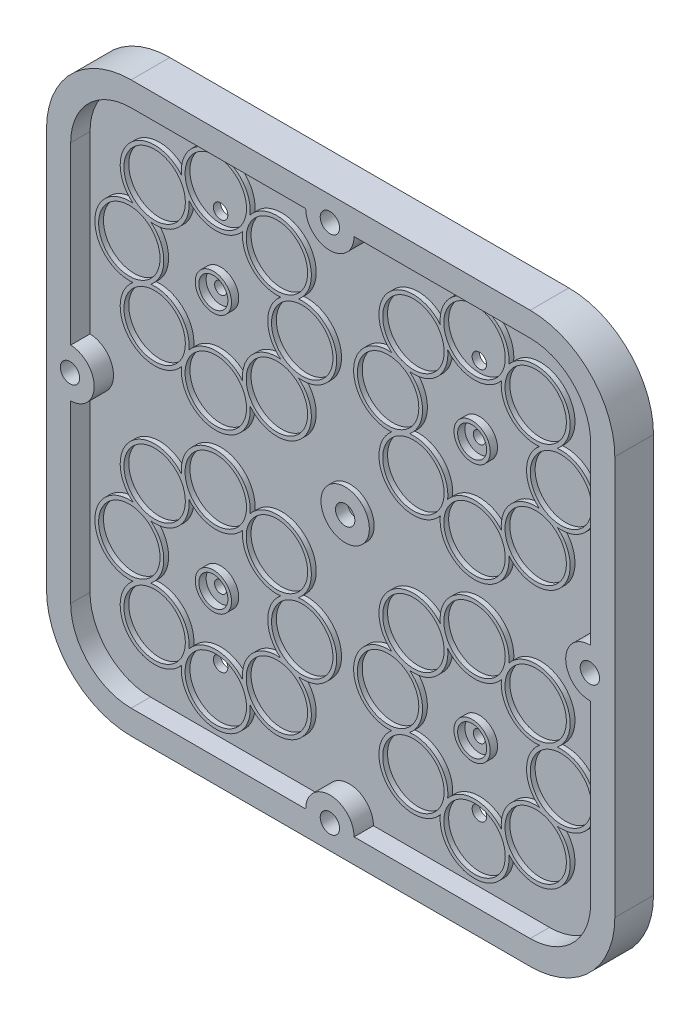
from build123d import *

# Parameters (mm, degrees)
SKETCH1_R           = 4
SKETCH1_R_2         = 2.5
BOSS_EXTRUDE1_DEPTH = 3
SKETCH2_R           = 4
BOSS_EXTRUDE2_DEPTH = 8
SKETCH3_R           = 10
SKETCH3_R_2         = 4
BOSS_EXTRUDE3_DEPTH = 2
SKETCH4_R           = 12.7
BOSS_EXTRUDE4_DEPTH = 2
SKETCH5_R           = 7.5
SKETCH5_R_2         = 6
BOSS_EXTRUDE5_DEPTH = 3
SKETCH6_R           = 3
CUT_EXTRUDE1_DEPTH  = 10
BOSS_EXTRUDE6_START = 4
SKETCH7_R           = 19
SKETCH7_R_2         = 7.5
BOSS_EXTRUDE6_DEPTH = 4
SKETCH8_R           = 14.5
SKETCH8_R_2         = 9.5
BOSS_EXTRUDE7_DEPTH = 6


with BuildPart() as part:
    # Sketch1 → Boss-Extrude1 (new body)
    with BuildSketch(Plane.XY):
        with BuildLine():
            Line((35, 0), (200, 0))
            ThreePointArc((200, 0), (224.748737342, 10.251262658), (235, 35))
            Line((235, 35), (235, 200))
            ThreePointArc((235, 200), (224.748737342, 224.748737342), (200, 235))
            Line((200, 235), (35, 235))
            ThreePointArc((35, 235), (10.251262658, 224.748737342), (0, 200))
            Line((0, 200), (0, 35))
            ThreePointArc((0, 35), (10.251262658, 10.251262658), (35, 0))
        make_face()
        with Locations((117.5, 225)):
            Circle(SKETCH1_R, mode=Mode.SUBTRACT)
        with Locations((117.5, 10)):
            Circle(SKETCH1_R, mode=Mode.SUBTRACT)
        with Locations((117.5, 117.5)):
            Circle(SKETCH1_R, mode=Mode.SUBTRACT)
        with Locations((225, 117.5)):
            Circle(SKETCH1_R, mode=Mode.SUBTRACT)
        with Locations((10, 117.5)):
            Circle(SKETCH1_R, mode=Mode.SUBTRACT)
        with Locations((64, 171)):
            Circle(SKETCH1_R_2, mode=Mode.SUBTRACT)
        with Locations((171, 171)):
            Circle(SKETCH1_R_2, mode=Mode.SUBTRACT)
        with Locations((171, 64)):
            Circle(SKETCH1_R_2, mode=Mode.SUBTRACT)
        with Locations((64, 64)):
            Circle(SKETCH1_R_2, mode=Mode.SUBTRACT)
    extrude(amount=BOSS_EXTRUDE1_DEPTH)

    # Sketch2 → Boss-Extrude2 (add, symmetric)
    with BuildSketch(Plane.XY.offset(3)):
        with BuildLine():
            Line((235, 35), (235, 200))
            ThreePointArc((235, 200), (224.748737342, 224.748737342), (200, 235))
            Line((200, 235), (35, 235))
            ThreePointArc((35, 235), (10.251262658, 224.748737342), (0, 200))
            Line((0, 200), (0, 35))
            ThreePointArc((0, 35), (10.251262658, 10.251262658), (35, 0))
            Line((35, 0), (200, 0))
            ThreePointArc((200, 0), (224.748737342, 10.251262658), (235, 35))
        make_face()
        with Locations((117.185983795, 225.007361775)):
            Circle(SKETCH2_R, mode=Mode.SUBTRACT)
        with Locations((224.685983795, 117.507361775)):
            Circle(SKETCH2_R, mode=Mode.SUBTRACT)
        with Locations((117.185983795, 10.007361775)):
            Circle(SKETCH2_R, mode=Mode.SUBTRACT)
        with Locations((9.72235037, 117.506509199)):
            Circle(SKETCH2_R, mode=Mode.SUBTRACT)
        with BuildLine():
            Line((200, 225), (127.185981085, 225))
            ThreePointArc((127.185981085, 225), (117.185983795, 215.007361775), (107.185986504, 225))
            Line((107.185986504, 225), (35, 225))
            ThreePointArc((35, 225), (17.32233047, 217.67766953), (10, 200))
            Line((10, 200), (10, 127.50265399))
            ThreePointArc((10, 127.50265399), (19.72235037, 117.506509199), (10, 107.510364408))
            Line((10, 107.510364408), (10, 35))
            ThreePointArc((10, 35), (17.32233047, 17.32233047), (35, 10))
            Line((35, 10), (107.185986504, 10))
            ThreePointArc((107.185986504, 10), (117.185983795, 20.007361775), (127.185981085, 10))
            Line((127.185981085, 10), (200, 10))
            ThreePointArc((200, 10), (217.67766953, 17.32233047), (225, 35))
            Line((225, 35), (225, 107.5122933))
            ThreePointArc((225, 107.5122933), (214.685983795, 117.507361775), (225, 127.50243025))
            Line((225, 127.50243025), (225, 200))
            ThreePointArc((225, 200), (217.67766953, 217.67766953), (200, 225))
        make_face(mode=Mode.SUBTRACT)
    extrude(amount=BOSS_EXTRUDE2_DEPTH, both=True)

    # Sketch3 → Boss-Extrude3 (add)
    with BuildSketch(Plane.XY.offset(3)):
        with Locations((117.5, 117.5)):
            Circle(SKETCH3_R)
        with Locations((117.5, 117.5)):
            Circle(SKETCH3_R_2, mode=Mode.SUBTRACT)
    extrude(amount=BOSS_EXTRUDE3_DEPTH)

    # Sketch4 → Boss-Extrude4 (add)
    # profile 1 of 4: a face of its own
    with BuildSketch(Plane.XY.offset(3)):
        with BuildLine():
            ThreePointArc((136.802142668, 185.165216311), (121, 171), (136.802142668, 156.834783689))
            ThreePointArc((136.802142668, 156.834783689), (135.644660941, 135.644660941), (156.834783689, 136.802142668))
            ThreePointArc((156.834783689, 136.802142668), (171, 121), (185.165216311, 136.802142668))
            ThreePointArc((185.165216311, 136.802142668), (206.355339059, 135.644660941), (205.197857332, 156.834783689))
            ThreePointArc((205.197857332, 156.834783689), (221, 171), (205.197857332, 185.165216311))
            ThreePointArc((205.197857332, 185.165216311), (206.355339059, 206.355339059), (185.165216311, 205.197857332))
            ThreePointArc((185.165216311, 205.197857332), (171, 221), (156.834783689, 205.197857332))
            ThreePointArc((156.834783689, 205.197857332), (135.644660941, 206.355339059), (136.802142668, 185.165216311))
        make_face()
        with Locations((171, 206.75)):
            Circle(SKETCH4_R, mode=Mode.SUBTRACT)
        with Locations((145.720932573, 196.279067427)):
            Circle(SKETCH4_R, mode=Mode.SUBTRACT)
        with Locations((135.25, 171)):
            Circle(SKETCH4_R, mode=Mode.SUBTRACT)
        with Locations((145.720932573, 145.720932573)):
            Circle(SKETCH4_R, mode=Mode.SUBTRACT)
        with Locations((171, 135.25)):
            Circle(SKETCH4_R, mode=Mode.SUBTRACT)
        with Locations((196.279067427, 145.720932573)):
            Circle(SKETCH4_R, mode=Mode.SUBTRACT)
        with Locations((206.75, 171)):
            Circle(SKETCH4_R, mode=Mode.SUBTRACT)
        with Locations((196.279067427, 196.279067427)):
            Circle(SKETCH4_R, mode=Mode.SUBTRACT)
        with BuildLine():
            ThreePointArc((159.886148884, 197.831210095), (171, 192.5), (182.113851116, 197.831210095))
            ThreePointArc((182.113851116, 197.831210095), (186.202795796, 186.202795796), (197.831210095, 182.113851116))
            ThreePointArc((197.831210095, 182.113851116), (192.5, 171), (197.831210095, 159.886148884))
            ThreePointArc((197.831210095, 159.886148884), (186.202795796, 155.797204204), (182.113851116, 144.168789905))
            ThreePointArc((182.113851116, 144.168789905), (171, 149.5), (159.886148884, 144.168789905))
            ThreePointArc((159.886148884, 144.168789905), (155.797204204, 155.797204204), (144.168789905, 159.886148884))
            ThreePointArc((144.168789905, 159.886148884), (149.5, 171), (144.168789905, 182.113851116))
            ThreePointArc((144.168789905, 182.113851116), (155.797204204, 186.202795796), (159.886148884, 197.831210095))
        make_face(mode=Mode.SUBTRACT)
    # profile 2 of 4: a face of its own
    with BuildSketch(Plane.XY.offset(3)):
        with BuildLine():
            ThreePointArc((185.165216311, 98.197857332), (171, 114), (156.834783689, 98.197857332))
            ThreePointArc((156.834783689, 98.197857332), (135.644660941, 99.355339059), (136.802142668, 78.165216311))
            ThreePointArc((136.802142668, 78.165216311), (121, 64), (136.802142668, 49.834783689))
            ThreePointArc((136.802142668, 49.834783689), (135.644660941, 28.644660941), (156.834783689, 29.802142668))
            ThreePointArc((156.834783689, 29.802142668), (171, 14), (185.165216311, 29.802142668))
            ThreePointArc((185.165216311, 29.802142668), (206.355339059, 28.644660941), (205.197857332, 49.834783689))
            ThreePointArc((205.197857332, 49.834783689), (221, 64), (205.197857332, 78.165216311))
            ThreePointArc((205.197857332, 78.165216311), (206.355339059, 99.355339059), (185.165216311, 98.197857332))
        make_face()
        with Locations((171, 99.75)):
            Circle(SKETCH4_R, mode=Mode.SUBTRACT)
        with Locations((145.720932573, 89.279067427)):
            Circle(SKETCH4_R, mode=Mode.SUBTRACT)
        with Locations((135.25, 64)):
            Circle(SKETCH4_R, mode=Mode.SUBTRACT)
        with Locations((145.720932573, 38.720932573)):
            Circle(SKETCH4_R, mode=Mode.SUBTRACT)
        with Locations((171, 28.25)):
            Circle(SKETCH4_R, mode=Mode.SUBTRACT)
        with Locations((196.279067427, 38.720932573)):
            Circle(SKETCH4_R, mode=Mode.SUBTRACT)
        with Locations((206.75, 64)):
            Circle(SKETCH4_R, mode=Mode.SUBTRACT)
        with Locations((196.279067427, 89.279067427)):
            Circle(SKETCH4_R, mode=Mode.SUBTRACT)
        with BuildLine():
            ThreePointArc((144.168789905, 75.113851116), (155.797204204, 79.202795796), (159.886148884, 90.831210095))
            ThreePointArc((159.886148884, 90.831210095), (171, 85.5), (182.113851116, 90.831210095))
            ThreePointArc((182.113851116, 90.831210095), (186.202795796, 79.202795796), (197.831210095, 75.113851116))
            ThreePointArc((197.831210095, 75.113851116), (192.5, 64), (197.831210095, 52.886148884))
            ThreePointArc((197.831210095, 52.886148884), (186.202795796, 48.797204204), (182.113851116, 37.168789905))
            ThreePointArc((182.113851116, 37.168789905), (171, 42.5), (159.886148884, 37.168789905))
            ThreePointArc((159.886148884, 37.168789905), (155.797204204, 48.797204204), (144.168789905, 52.886148884))
            ThreePointArc((144.168789905, 52.886148884), (149.5, 64), (144.168789905, 75.113851116))
        make_face(mode=Mode.SUBTRACT)
    # profile 3 of 4: a face of its own
    with BuildSketch(Plane.XY.offset(3)):
        with BuildLine():
            ThreePointArc((98.197857332, 49.834783689), (114, 64), (98.197857332, 78.165216311))
            ThreePointArc((98.197857332, 78.165216311), (99.355339059, 99.355339059), (78.165216311, 98.197857332))
            ThreePointArc((78.165216311, 98.197857332), (64, 114), (49.834783689, 98.197857332))
            ThreePointArc((49.834783689, 98.197857332), (28.644660941, 99.355339059), (29.802142668, 78.165216311))
            ThreePointArc((29.802142668, 78.165216311), (14, 64), (29.802142668, 49.834783689))
            ThreePointArc((29.802142668, 49.834783689), (28.644660941, 28.644660941), (49.834783689, 29.802142668))
            ThreePointArc((49.834783689, 29.802142668), (64, 14), (78.165216311, 29.802142668))
            ThreePointArc((78.165216311, 29.802142668), (99.355339059, 28.644660941), (98.197857332, 49.834783689))
        make_face()
        with Locations((99.75, 64)):
            Circle(SKETCH4_R, mode=Mode.SUBTRACT)
        with Locations((89.279067427, 89.279067427)):
            Circle(SKETCH4_R, mode=Mode.SUBTRACT)
        with Locations((64, 99.75)):
            Circle(SKETCH4_R, mode=Mode.SUBTRACT)
        with Locations((38.720932573, 89.279067427)):
            Circle(SKETCH4_R, mode=Mode.SUBTRACT)
        with Locations((28.25, 64)):
            Circle(SKETCH4_R, mode=Mode.SUBTRACT)
        with Locations((38.720932573, 38.720932573)):
            Circle(SKETCH4_R, mode=Mode.SUBTRACT)
        with Locations((64, 28.25)):
            Circle(SKETCH4_R, mode=Mode.SUBTRACT)
        with Locations((89.279067427, 38.720932573)):
            Circle(SKETCH4_R, mode=Mode.SUBTRACT)
        with BuildLine():
            ThreePointArc((75.113851116, 90.831210095), (79.202795796, 79.202795796), (90.831210095, 75.113851116))
            ThreePointArc((90.831210095, 75.113851116), (85.5, 64), (90.831210095, 52.886148884))
            ThreePointArc((90.831210095, 52.886148884), (79.202795796, 48.797204204), (75.113851116, 37.168789905))
            ThreePointArc((75.113851116, 37.168789905), (64, 42.5), (52.886148884, 37.168789905))
            ThreePointArc((52.886148884, 37.168789905), (48.797204204, 48.797204204), (37.168789905, 52.886148884))
            ThreePointArc((37.168789905, 52.886148884), (42.5, 64), (37.168789905, 75.113851116))
            ThreePointArc((37.168789905, 75.113851116), (48.797204204, 79.202795796), (52.886148884, 90.831210095))
            ThreePointArc((52.886148884, 90.831210095), (64, 85.5), (75.113851116, 90.831210095))
        make_face(mode=Mode.SUBTRACT)
    # profile 4 of 4: a face of its own
    with BuildSketch(Plane.XY.offset(3)):
        with BuildLine():
            ThreePointArc((49.834783689, 136.802142668), (64, 121), (78.165216311, 136.802142668))
            ThreePointArc((78.165216311, 136.802142668), (99.355339059, 135.644660941), (98.197857332, 156.834783689))
            ThreePointArc((98.197857332, 156.834783689), (114, 171), (98.197857332, 185.165216311))
            ThreePointArc((98.197857332, 185.165216311), (99.355339059, 206.355339059), (78.165216311, 205.197857332))
            ThreePointArc((78.165216311, 205.197857332), (64, 221), (49.834783689, 205.197857332))
            ThreePointArc((49.834783689, 205.197857332), (28.644660941, 206.355339059), (29.802142668, 185.165216311))
            ThreePointArc((29.802142668, 185.165216311), (14, 171), (29.802142668, 156.834783689))
            ThreePointArc((29.802142668, 156.834783689), (28.644660941, 135.644660941), (49.834783689, 136.802142668))
        make_face()
        with Locations((64, 135.25)):
            Circle(SKETCH4_R, mode=Mode.SUBTRACT)
        with Locations((89.279067427, 145.720932573)):
            Circle(SKETCH4_R, mode=Mode.SUBTRACT)
        with Locations((99.75, 171)):
            Circle(SKETCH4_R, mode=Mode.SUBTRACT)
        with Locations((89.279067427, 196.279067427)):
            Circle(SKETCH4_R, mode=Mode.SUBTRACT)
        with Locations((64, 206.75)):
            Circle(SKETCH4_R, mode=Mode.SUBTRACT)
        with Locations((38.720932573, 196.279067427)):
            Circle(SKETCH4_R, mode=Mode.SUBTRACT)
        with Locations((28.25, 171)):
            Circle(SKETCH4_R, mode=Mode.SUBTRACT)
        with Locations((38.720932573, 145.720932573)):
            Circle(SKETCH4_R, mode=Mode.SUBTRACT)
        with BuildLine():
            ThreePointArc((90.831210095, 159.886148884), (79.202795796, 155.797204204), (75.113851116, 144.168789905))
            ThreePointArc((75.113851116, 144.168789905), (64, 149.5), (52.886148884, 144.168789905))
            ThreePointArc((52.886148884, 144.168789905), (48.797204204, 155.797204204), (37.168789905, 159.886148884))
            ThreePointArc((37.168789905, 159.886148884), (42.5, 171), (37.168789905, 182.113851116))
            ThreePointArc((37.168789905, 182.113851116), (48.797204204, 186.202795796), (52.886148884, 197.831210095))
            ThreePointArc((52.886148884, 197.831210095), (64, 192.5), (75.113851116, 197.831210095))
            ThreePointArc((75.113851116, 197.831210095), (79.202795796, 186.202795796), (90.831210095, 182.113851116))
            ThreePointArc((90.831210095, 182.113851116), (85.5, 171), (90.831210095, 159.886148884))
        make_face(mode=Mode.SUBTRACT)
    extrude(amount=BOSS_EXTRUDE4_DEPTH)

    # Sketch5 → Boss-Extrude5 (add)
    # profile 1 of 4: a face of its own
    with BuildSketch(Plane.XY.offset(3)):
        with Locations((171, 171)):
            Circle(SKETCH5_R)
        with Locations((171, 171)):
            Circle(SKETCH5_R_2, mode=Mode.SUBTRACT)
    # profile 2 of 4: a face of its own
    with BuildSketch(Plane.XY.offset(3)):
        with Locations((64, 171)):
            Circle(SKETCH5_R)
        with Locations((64, 171)):
            Circle(SKETCH5_R_2, mode=Mode.SUBTRACT)
    # profile 3 of 4: a face of its own
    with BuildSketch(Plane.XY.offset(3)):
        with Locations((64, 64)):
            Circle(SKETCH5_R)
        with Locations((64, 64)):
            Circle(SKETCH5_R_2, mode=Mode.SUBTRACT)
    # profile 4 of 4: a face of its own
    with BuildSketch(Plane.XY.offset(3)):
        with Locations((171, 64)):
            Circle(SKETCH5_R)
        with Locations((171, 64)):
            Circle(SKETCH5_R_2, mode=Mode.SUBTRACT)
    extrude(amount=BOSS_EXTRUDE5_DEPTH)

    # Sketch6 → Cut-Extrude1 (cut)
    with BuildSketch(Plane(origin=(0, 0, 0), x_dir=(-1, 0, 0), z_dir=(0, 0, -1))):
        with Locations((-64, 36.5)):
            Circle(SKETCH6_R)
        with Locations((-171, 36.5)):
            Circle(SKETCH6_R)
        with Locations((-171, 198.5)):
            Circle(SKETCH6_R)
        with Locations((-64, 198.5)):
            Circle(SKETCH6_R)
    extrude(amount=-CUT_EXTRUDE1_DEPTH, mode=Mode.SUBTRACT)

    # Sketch7 → Boss-Extrude6 (add)
    # profile 1 of 4: a face of its own
    with BuildSketch(Plane(origin=(0, 0, 0), x_dir=(-1, 0, 0), z_dir=(0, 0, -1)).offset(BOSS_EXTRUDE6_START)):
        with BuildLine():
            ThreePointArc((-177.977271247, 56.836363636), (-171, 15), (-164.022728753, 56.836363636))
            ThreePointArc((-164.022728753, 56.836363636), (-171, 74), (-177.977271247, 56.836363636))
        make_face()
        with Locations((-171, 36.5)):
            Circle(SKETCH7_R, mode=Mode.SUBTRACT)
        with Locations(Location((-171, 64, 0), (0, 0, 180))):
            Circle(SKETCH7_R_2, mode=Mode.SUBTRACT)
    # profile 2 of 4: a face of its own
    with BuildSketch(Plane(origin=(0, 0, 0), x_dir=(-1, 0, 0), z_dir=(0, 0, -1)).offset(BOSS_EXTRUDE6_START)):
        with BuildLine():
            ThreePointArc((-70.977271247, 56.836363636), (-64, 74), (-57.022728753, 56.836363636))
            ThreePointArc((-57.022728753, 56.836363636), (-64, 15), (-70.977271247, 56.836363636))
        make_face()
        with Locations(Location((-64, 64, 0), (0, 0, 180))):
            Circle(SKETCH7_R_2, mode=Mode.SUBTRACT)
        with Locations(Location((-64, 36.5, 0), (0, 0, 180))):
            Circle(SKETCH7_R, mode=Mode.SUBTRACT)
    # profile 3 of 4: a face of its own
    with BuildSketch(Plane(origin=(0, 0, 0), x_dir=(-1, 0, 0), z_dir=(0, 0, -1)).offset(BOSS_EXTRUDE6_START)):
        with BuildLine():
            ThreePointArc((-164.022728753, 178.163636364), (-171, 161), (-177.977271247, 178.163636364))
            ThreePointArc((-177.977271247, 178.163636364), (-171, 220), (-164.022728753, 178.163636364))
        make_face()
        with Locations(Location((-171, 171, 0), (0, 0, 180))):
            Circle(SKETCH7_R_2, mode=Mode.SUBTRACT)
        with Locations(Location((-171, 198.5, 0), (0, 0, 180))):
            Circle(SKETCH7_R, mode=Mode.SUBTRACT)
    # profile 4 of 4: a face of its own
    with BuildSketch(Plane(origin=(0, 0, 0), x_dir=(-1, 0, 0), z_dir=(0, 0, -1)).offset(BOSS_EXTRUDE6_START)):
        with BuildLine():
            ThreePointArc((-57.022728753, 178.163636364), (-64, 220), (-70.977271247, 178.163636364))
            ThreePointArc((-70.977271247, 178.163636364), (-64, 161), (-57.022728753, 178.163636364))
        make_face()
        with Locations((-64, 198.5)):
            Circle(SKETCH7_R, mode=Mode.SUBTRACT)
        with Locations(Location((-64, 171, 0), (0, 0, 180))):
            Circle(SKETCH7_R_2, mode=Mode.SUBTRACT)
    extrude(amount=-BOSS_EXTRUDE6_DEPTH)

    # Sketch8 → Boss-Extrude7 (add)
    with BuildSketch(Plane(origin=(0, 0, 0), x_dir=(-1, 0, 0), z_dir=(0, 0, -1))):
        with Locations(Location((-117.5, 117.5, 0), (0, 0, 180))):
            Circle(SKETCH8_R)
        with Locations((-117.5, 117.5)):
            Circle(SKETCH8_R_2, mode=Mode.SUBTRACT)
    extrude(amount=BOSS_EXTRUDE7_DEPTH)


solid = part.part
